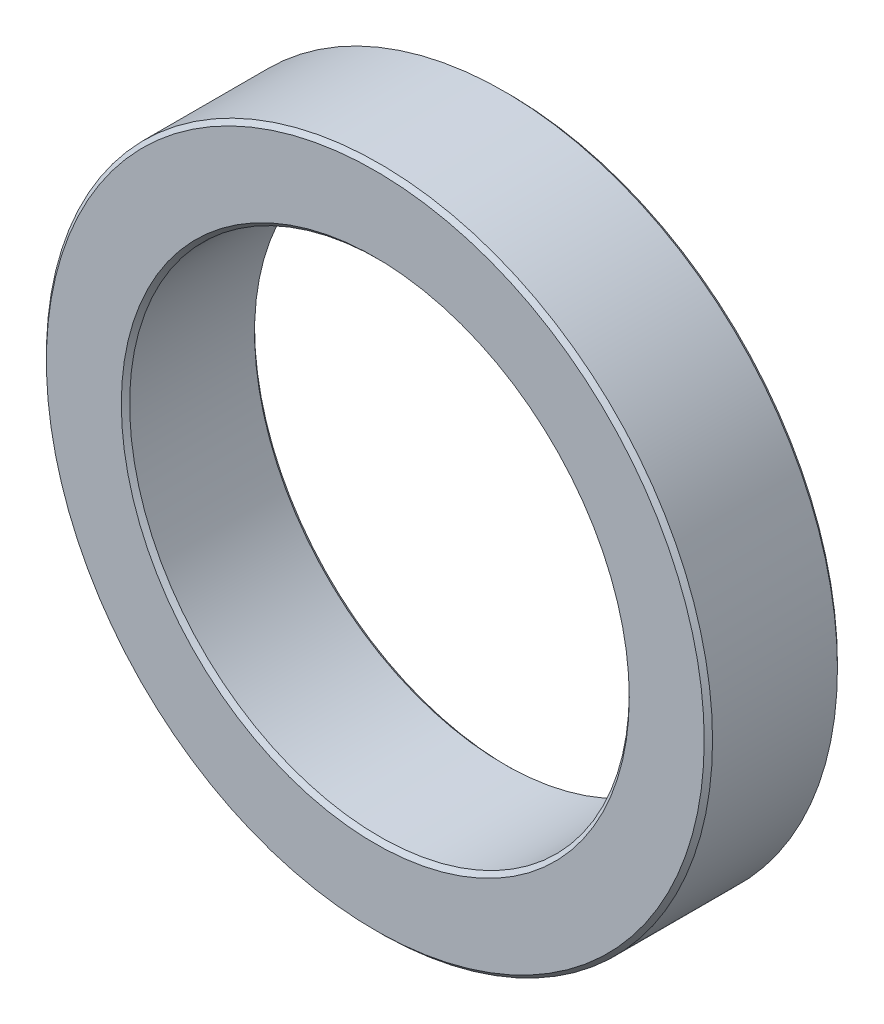
SolidWorks part; units mm, degrees
ref_plane "Front Plane" through (0, 0, 0) normal (0, 0, 1) x (1, 0, 0)
ref_plane "Top Plane" through (0, 0, 0) normal (0, 1, 0) x (1, 0, 0)
ref_plane "Right Plane" through (0, 0, 0) normal (1, 0, 0) x (0, 0, -1)
sketch "Sketch1" plane through (0, 0, 0) normal (0, 0, 1) x (1, 0, 0)
  circle A0 centre (0, 0) radius 30
  circle A1 centre (0, 0) radius 40
  dimension "D1" = 80
  dimension "D2" = 60
extrude "Boss-Extrude1" add sketch "Sketch1" along normal blind 16
chamfer "Chamfer1" distance 0.5 angle 45 4 edges at (30, 0, 0) (40, 0, 0) (30, 0, 16) (40, 0, 16)
